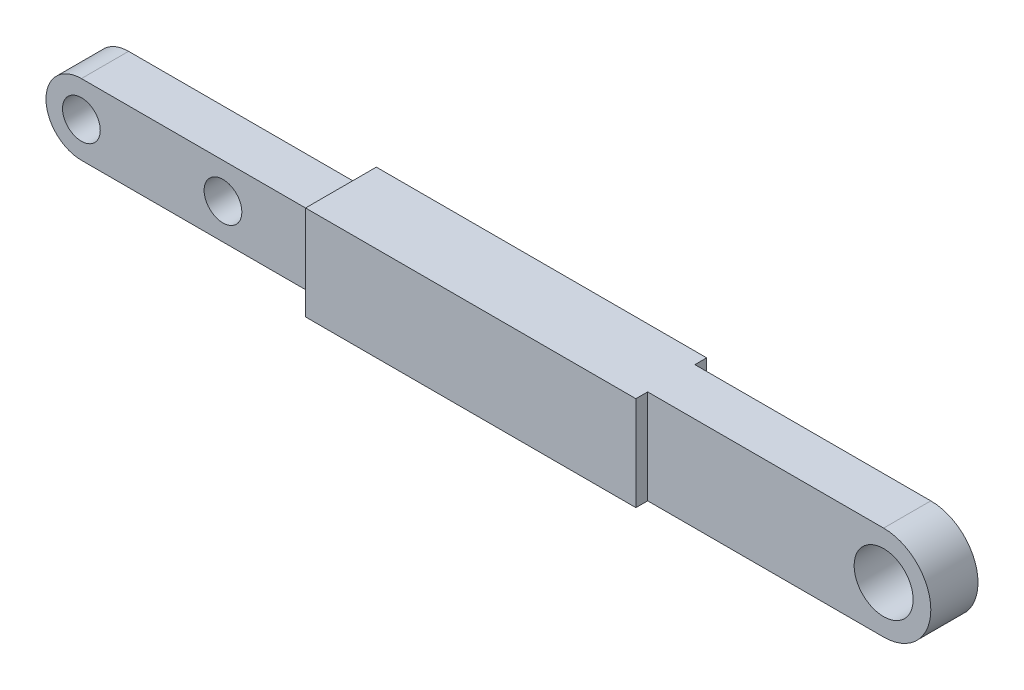
from build123d import *

# Parameters (mm, degrees)
SKETCH1_R           = 0.625
BOSS_EXTRUDE1_DEPTH = 0.75
SKETCH3_R           = 0.4
BOSS_EXTRUDE3_DEPTH = 0.5
CUT_EXTRUDE1_START  = -0.25
CUT_EXTRUDE1_DEPTH  = 0.25


with BuildPart() as part:
    # Sketch1 → Boss-Extrude1 (new, symmetric)
    with BuildSketch(Plane.XY):
        with BuildLine():
            Line((0, -1), (0, 1))
            Line((0, 1), (12, 1))
            ThreePointArc((12, 1), (13, 0), (12, -1))
            Line((12, -1), (0, -1))
        make_face()
        with Locations((12, 0)):
            Circle(SKETCH1_R, mode=Mode.SUBTRACT)
    extrude(amount=BOSS_EXTRUDE1_DEPTH, both=True)

    # Sketch3 → Boss-Extrude3 (add, symmetric)
    with BuildSketch(Plane.XY):
        with BuildLine():
            Line((0, -0.75), (-5, -0.75))
            ThreePointArc((-5, -0.75), (-5.75, 0), (-5, 0.75))
            Line((-5, 0.75), (0, 0.75))
            Line((0, 0.75), (0, -0.75))
        make_face()
        with Locations((-5, 0)):
            Circle(SKETCH3_R, mode=Mode.SUBTRACT)
        with Locations((-2, 0)):
            Circle(SKETCH3_R, mode=Mode.SUBTRACT)
    extrude(amount=BOSS_EXTRUDE3_DEPTH, both=True)

    # Sketch6 → Cut-Extrude1 (cut)
    with BuildSketch(Plane(origin=(0, 0, -0.75), x_dir=(-1, 0, 0), z_dir=(0, 0, -1)).offset(CUT_EXTRUDE1_START)):
        with BuildLine():
            Line((-7, 1), (-7, -1))
            Line((-7, -1), (-12, -1))
            ThreePointArc((-12, -1), (-13, 0), (-12, 1))
            Line((-12, 1), (-7, 1))
        make_face()
    cut_extrude1 = extrude(amount=CUT_EXTRUDE1_DEPTH, mode=Mode.SUBTRACT)

    # Mirror1: Cut-Extrude1 across plane
    add(cut_extrude1.mirror(Plane.XY), mode=Mode.SUBTRACT)


solid = part.part
